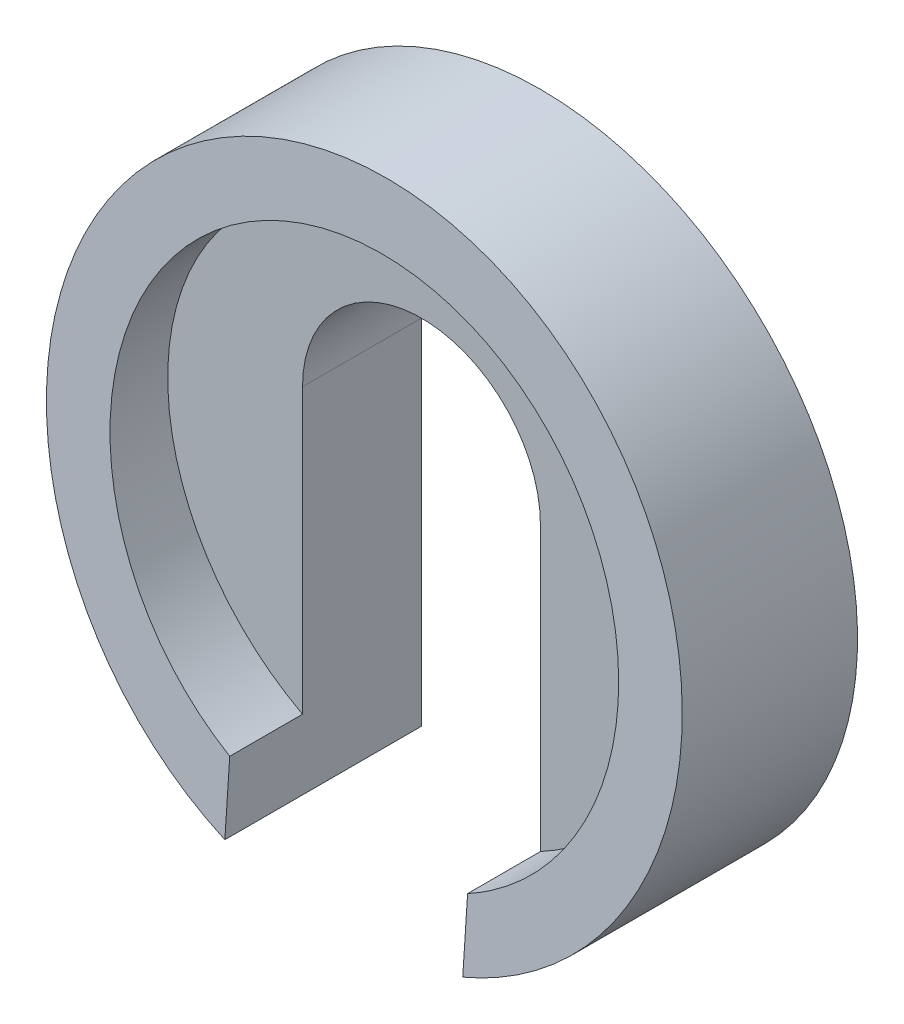
from build123d import *

# Parameters (mm, degrees)
CUT_EXTRUDE1_DEPTH      = 124.693168769
CUT_EXTRUDE1_DEPTH_BACK = 124.693168769
CUT_EXTRUDE2_DEPTH      = 124.693168769


with BuildPart() as part:
    # Sketch1 → Revolve2 (revolve)
    with BuildSketch(Plane(origin=(0, 0, 0), x_dir=(0, 0, -1), z_dir=(1, 0, 0))):
        Polygon((-50, 64), (-50, 80), (0, 80), (0, 0), (-30, 0), (-30, 64), align=None)
    revolve(axis=Axis((0, 0, -85.976986238), (0, 0, 1)))

    # Sketch2 → Cut-Extrude1 (cut, two sides: drawn at the far end of the back side and taken through both)
    with BuildSketch(Plane(origin=(0, 0, 0), x_dir=(0, 0, -1), z_dir=(1, 0, 0)).offset(-CUT_EXTRUDE1_DEPTH_BACK)):
        Polygon((-50, 80), (-38.811710089, 80), (-50, -80), align=None)
    extrude(amount=CUT_EXTRUDE1_DEPTH + CUT_EXTRUDE1_DEPTH_BACK, mode=Mode.SUBTRACT)

    # Sketch3 → Cut-Extrude2 (cut, through all)
    with BuildSketch(Plane.XY):
        with BuildLine():
            Line((30, 15), (30, -100))
            ThreePointArc((30, -100), (0, -130), (-30, -100))
            Line((-30, -100), (-30, 15))
            ThreePointArc((-30, 15), (0, 45), (30, 15))
        make_face()
    extrude(amount=CUT_EXTRUDE2_DEPTH, mode=Mode.SUBTRACT)


solid = part.part
